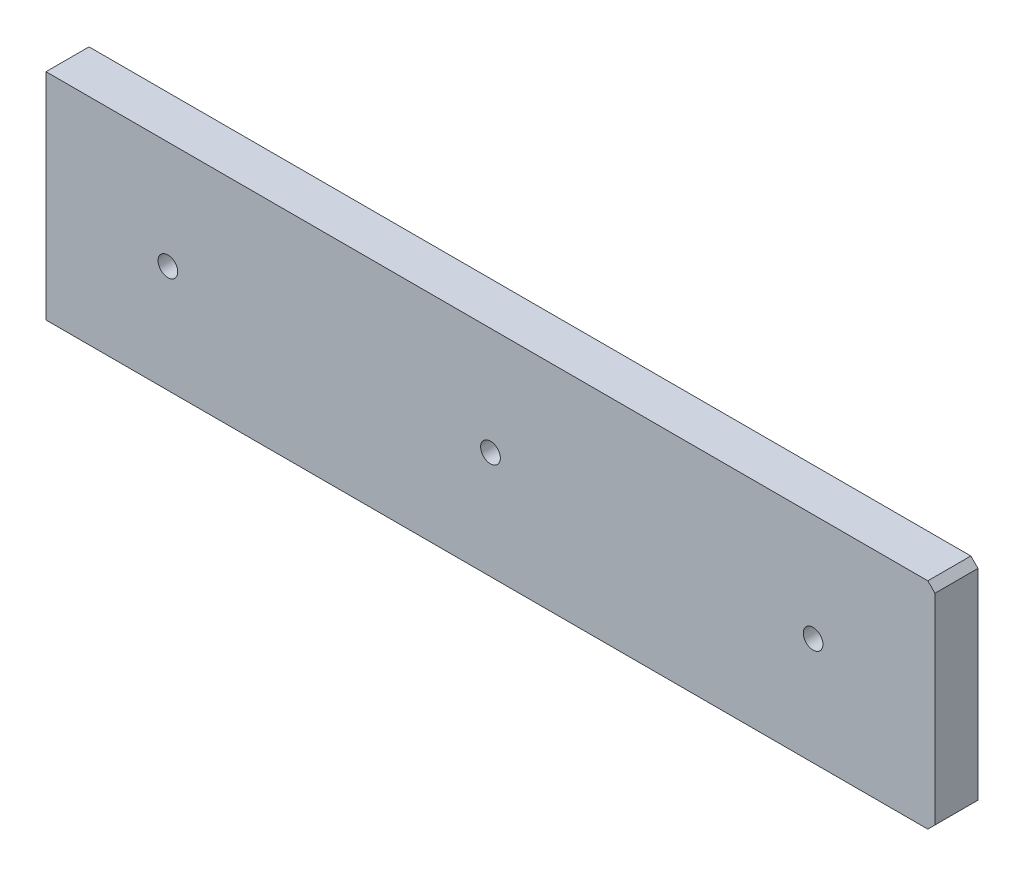
from build123d import *

# Parameters (mm, degrees)
SKETCH_1_W                     = 248
SKETCH_1_H                     = 60
EXTRUDE_1_DEPTH                = 6
HOLE_WIZARD_M5_1_D             = 4.2
HOLE_WIZARD_M5_1_DEPTH         = 12.4
HOLE_WIZARD_M5_1_TIP           = 1.2618073
CHAMFER_1_SIZE                 = 2
HOLE_WIZARD_M5_1_2_D           = 5.5
HOLE_WIZARD_M5_1_2_DEPTH       = 12.4
HOLE_WIZARD_M5_1_2_CBORE_D     = 10
HOLE_WIZARD_M5_1_2_CBORE_DEPTH = 5.7
HOLE_WIZARD_M5_1_2_TIP         = 1.652366702


with BuildPart() as part:
    # 草图1 → 凸台-拉伸1 (new, symmetric)
    with BuildSketch(Plane.XY):
        Rectangle(SKETCH_1_W, SKETCH_1_H)
    extrude(amount=EXTRUDE_1_DEPTH, both=True)

    # Hole Wizard M5 _1
    with Locations(Plane.ZY.offset(124)):
        with Locations((0, 20), (0, -20)):
            Hole(HOLE_WIZARD_M5_1_D / 2, depth=HOLE_WIZARD_M5_1_DEPTH)
            with Locations((0, 0, -(HOLE_WIZARD_M5_1_DEPTH + HOLE_WIZARD_M5_1_TIP / 2))):  # 118° drill point
                Cone(0, HOLE_WIZARD_M5_1_D / 2, HOLE_WIZARD_M5_1_TIP, mode=Mode.SUBTRACT)

    # 倒角1
    chamfer_1_edges = [part.edges().sort_by_distance(p)[0] for p in [
        (124, -30, 0),
        (124, 30, 0),
    ]]
    chamfer(chamfer_1_edges, length=CHAMFER_1_SIZE)

    # Hole Wizard M5 _1 2
    with Locations(Plane(origin=(0, 0, -6), x_dir=(-1, 0, 0), z_dir=(0, 0, -1))):
        with Locations((-90, 0), (0, 0), (90, 0)):
            CounterBoreHole(HOLE_WIZARD_M5_1_2_D / 2, HOLE_WIZARD_M5_1_2_CBORE_D / 2, HOLE_WIZARD_M5_1_2_CBORE_DEPTH, depth=HOLE_WIZARD_M5_1_2_DEPTH)
            with Locations((0, 0, -(HOLE_WIZARD_M5_1_2_DEPTH + HOLE_WIZARD_M5_1_2_TIP / 2))):  # 118° drill point
                Cone(0, HOLE_WIZARD_M5_1_2_D / 2, HOLE_WIZARD_M5_1_2_TIP, mode=Mode.SUBTRACT)


solid = part.part
